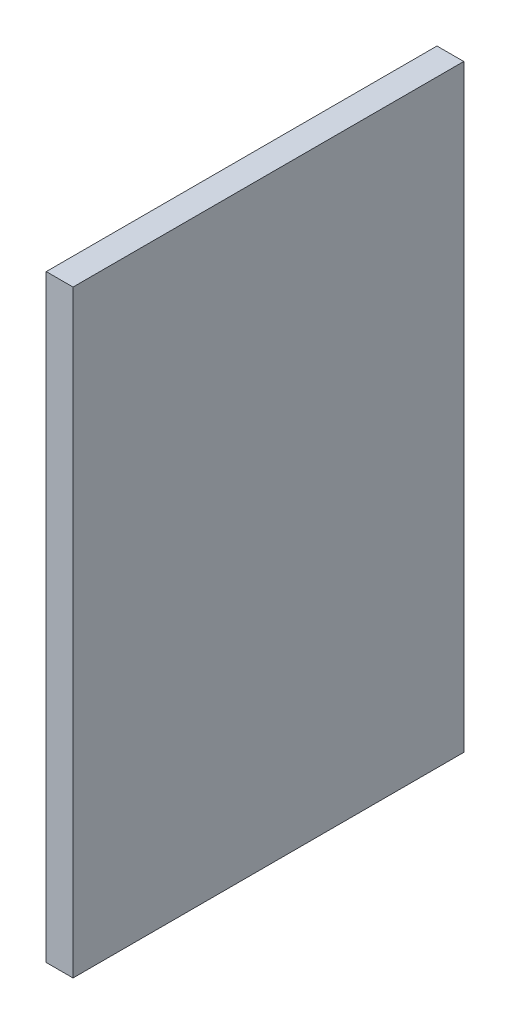
from build123d import *

# Parameters (mm, degrees)
SKETCH1_W           = 175
SKETCH1_H           = 268
BOSS_EXTRUDE1_DEPTH = 12


with BuildPart() as part:
    # Sketch1 → Boss-Extrude1 (new body)
    with BuildSketch(Plane(origin=(0, 0, 0), x_dir=(0, 0, -1), z_dir=(1, 0, 0))):
        with Locations((87.5, 134)):
            Rectangle(SKETCH1_W, SKETCH1_H)
    extrude(amount=BOSS_EXTRUDE1_DEPTH)


solid = part.part
